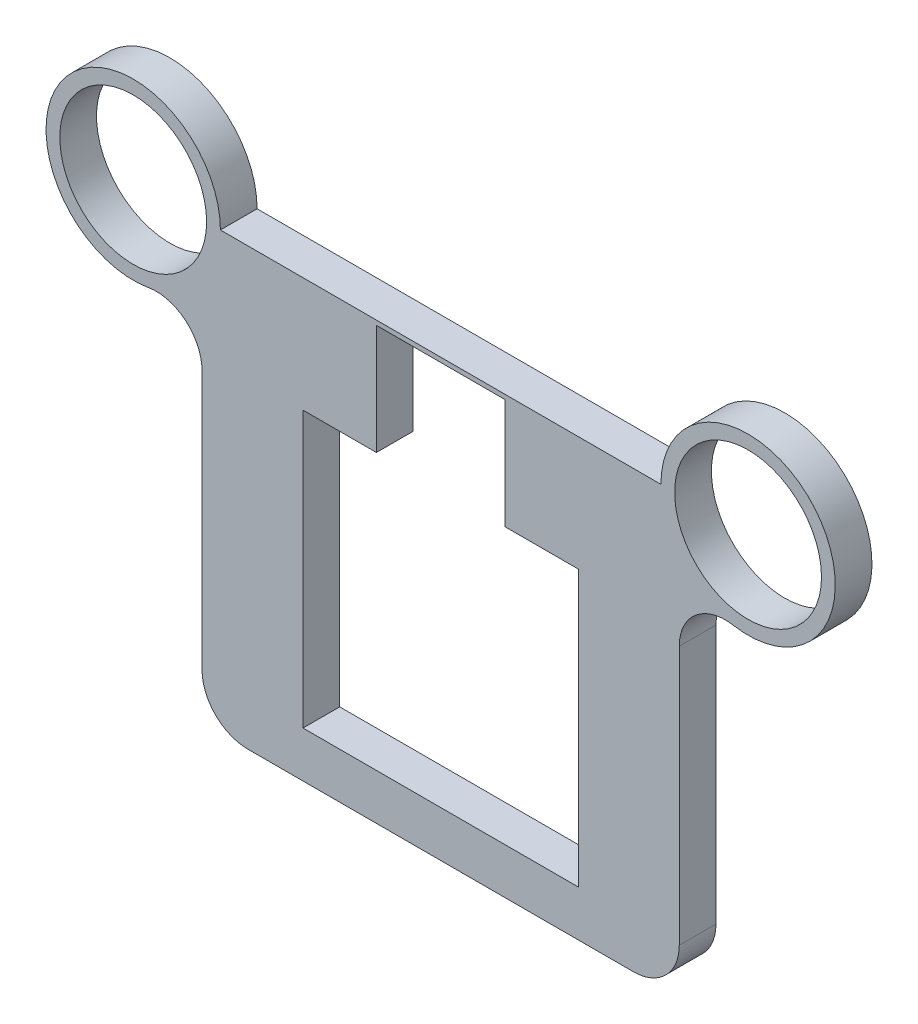
from build123d import *

# Parameters (mm, degrees)
SKETCH_1_R      = 16
EXTRUDE_1_DEPTH = 8


with BuildPart() as part:
    # 草图1 → 凸台-拉伸1 (new body)
    with BuildSketch(Plane.XY):
        with BuildLine():
            ThreePointArc((63.331817296, 16.731279855), (81.154867742, 47.668830358), (47.607679365, 35.446747461))
            Line((47.607679365, 35.446747461), (-47.607679365, 35.446747461))
            Line((-47.607679365, 35.446747461), (-48.392320635, 35.446747461))
            ThreePointArc((-48.392320635, 35.446747461), (-81.939509011, 47.668830358), (-64.116458566, 16.731279855))
            ThreePointArc((-64.116458566, 16.731279855), (-55.959645426, 14.537448682), (-52.392320635, 6.881033747))
            Line((-52.392320635, 6.881033747), (-52.392320635, -49.553252539))
            ThreePointArc((-52.392320635, -49.553252539), (-49.463388447, -56.624320351), (-42.392320635, -59.553252539))
            Line((-42.392320635, -59.553252539), (41.607679365, -59.553252539))
            ThreePointArc((41.607679365, -59.553252539), (48.678747177, -56.624320351), (51.607679365, -49.553252539))
            Line((51.607679365, -49.553252539), (51.607679365, 6.881033747))
            ThreePointArc((51.607679365, 6.881033747), (55.175004156, 14.537448682), (63.331817296, 16.731279855))
        make_face()
        Polygon((19.522836201, -49.553252539), (-28.363655741, -49.553252539), (-30.392320635, -49.553252539), (-30.392320635, 10.446747461), (-14.392320635, 10.446747461), (-14.392320635, 34.446747461), (13.607679365, 34.446747461), (13.607679365, 10.446747461), (29.607679365, 10.446747461), (29.607679365, -49.553252539), align=None, mode=Mode.SUBTRACT)
        with Locations((-67.392320635, 35.446747461)):
            Circle(SKETCH_1_R, mode=Mode.SUBTRACT)
        with Locations((66.607679365, 35.446747461)):
            Circle(SKETCH_1_R, mode=Mode.SUBTRACT)
    extrude(amount=EXTRUDE_1_DEPTH)


solid = part.part
